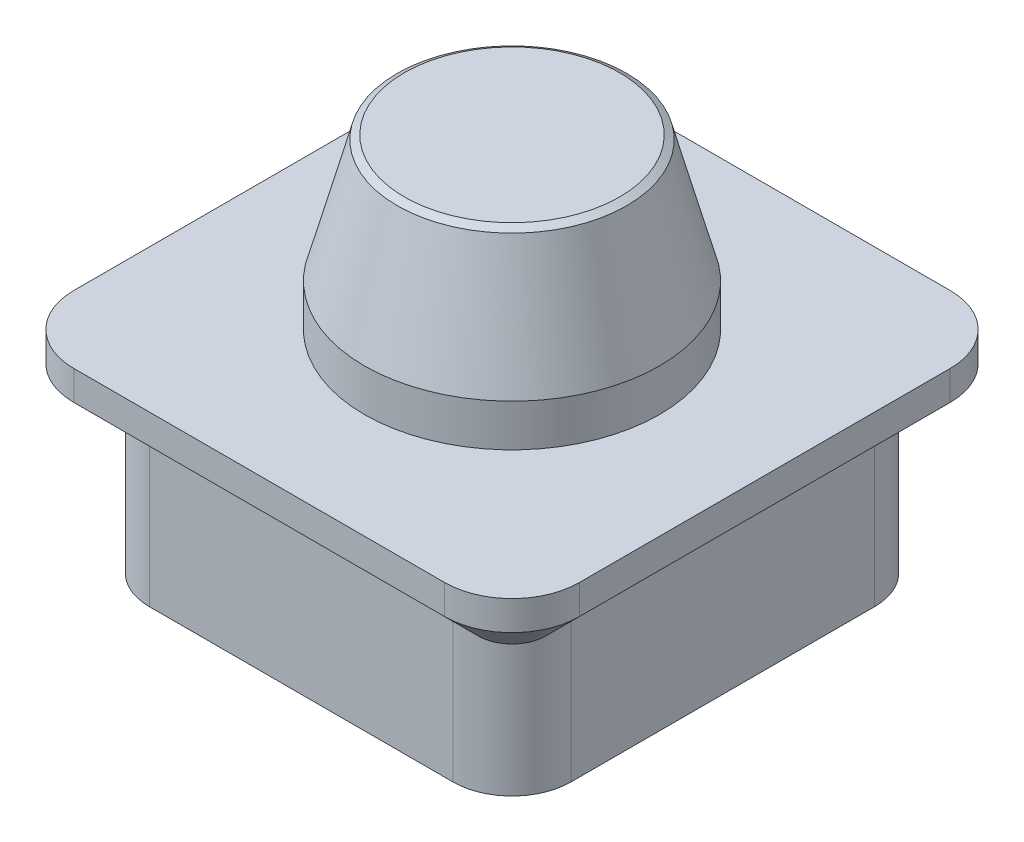
SolidWorks part; units mm, degrees
material "Q235B"
ref_plane "Front Plane" through (0, 0, 0) normal (0, 0, 1) x (1, 0, 0)
ref_plane "Top Plane" through (0, 0, 0) normal (0, 1, 0) x (1, 0, 0)
ref_plane "Right Plane" through (0, 0, 0) normal (1, 0, 0) x (0, 0, -1)
sketch "Sketch1" plane through (0, 0, 0) normal (0, 0, 1) x (1, 0, 0)
  line L0 (0, 0) -> (35, 0)
  line L1 (35, 0) -> (35, 10)
  line L2 (35, 10) -> (26.9615, 40)
  line L3 (26.9615, 40) -> (0, 40)
  line L4 (0, 40) -> (0, -18.6749) construction
  line L5 (0, 0) -> (0, 40)
  dimension "D1" = 70
  dimension "D2" = 15
  dimension "D3" = 10
  dimension "D4" = 40
revolve "Revolve1" add sketch "Sketch1" angle 360 about L4
chamfer "Chamfer1" distance 1 angle 45 1 edges at (-26.9615, 40, 0)
sketch "Sketch2" plane through (0, 0, 0) normal (0, -1, 0) x (1, 0, 0)
  line L1 (44, -60) -> (-44, -60)
  line L2 (60, -44) -> (60, 44)
  line L3 (44, 60) -> (-44, 60)
  line L4 (-60, -44) -> (-60, 44)
  line L5 (60, -60) -> (-60, 60) construction
  line L6 (60, 60) -> (-60, -60) construction
  arc A0 (-44, -60) -> (-60, -44) centre (-44, -44) cw
  arc A1 (60, 44) -> (44, 60) centre (44, 44) ccw
  arc A2 (44, -60) -> (60, -44) centre (44, -44) ccw
  arc A3 (-44, 60) -> (-60, 44) centre (-44, 44) ccw
  point P0 (0, 0)
  dimension "D2" = 16
  dimension "D1" = 120
extrude "Boss-Extrude1" add sketch "Sketch2" along normal blind 15
sketch "Sketch3" plane through (0, -15, 0) normal (0, -1, 0) x (1, 0, 0)
  line L1 (36, -50) -> (-36, -50)
  line L2 (50, -36) -> (50, 36)
  line L3 (36, 50) -> (-36, 50)
  line L4 (-50, -36) -> (-50, 36)
  line L5 (50, -50) -> (-50, 50) construction
  line L6 (50, 50) -> (-50, -50) construction
  arc A0 (-36, -50) -> (-50, -36) centre (-36, -36) cw
  arc A1 (50, 36) -> (36, 50) centre (36, 36) ccw
  arc A2 (36, -50) -> (50, -36) centre (36, -36) ccw
  arc A3 (-36, 50) -> (-50, 36) centre (-36, 36) ccw
  point P0 (0, 0)
  dimension "D2" = 14
  dimension "D1" = 100
extrude "Boss-Extrude2" add sketch "Sketch3" along normal blind 35
chamfer "Chamfer2" distance 8 angle 45 8 edges at (-55.3137, -15, -55.3137) (0, -15, -60) (-60, -15, 0) (55.3137, -15, -55.3137) (-55.3137, -15, 55.3137) (60, -15, 0) (0, -15, 60) (55.3137, -15, 55.3137)
